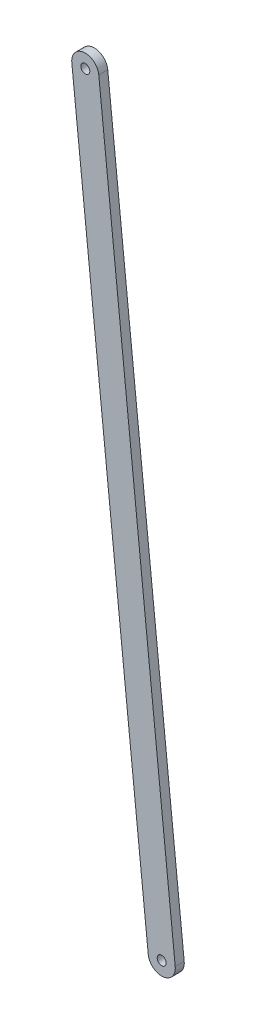
SolidWorks part; units mm, degrees
ref_plane "Front Plane" through (0, 0, 0) normal (0, 0, 1) x (1, 0, 0)
ref_plane "Top Plane" through (0, 0, 0) normal (0, 1, 0) x (1, 0, 0)
ref_plane "Right Plane" through (0, 0, 0) normal (1, 0, 0) x (0, 0, -1)
other "Configuration Table"
sketch "Sketch3" plane through (0, 0, 0) normal (0, 0, 1) x (1, 0, 0)
  line L0 (0, 793.0277) -> (0, 803.0277) construction
  line L1 (-15, 796.4658) -> (70, -19.8021)
  line L2 (70, 40) -> (70, -79.6043) construction
  line L4 (100, -79.6043) -> (100, 40) construction
  line L5 (100, -16.6782) -> (15, 799.5897)
  arc A0 (47.5615, 770.7422) -> (-47.5615, 770.7422) centre (0, 731.1325) ccw construction
  arc A1 (53.5752, 779.0765) -> (-53.5752, 779.0765) centre (0, 731.1325) ccw construction
  circle A3 centre (0, 798.0277) radius 5
  arc A4 (15, 799.5897) -> (-15, 796.4658) centre (0, 798.0277) ccw
  arc A5 (70, -19.8021) -> (100, -16.6782) centre (85, -18.2402) ccw
  circle A6 centre (85, -18.2402) radius 5
  dimension "D1" = 360
extrude "Boss-Extrude1" add sketch "Sketch3" along normal blind 10
